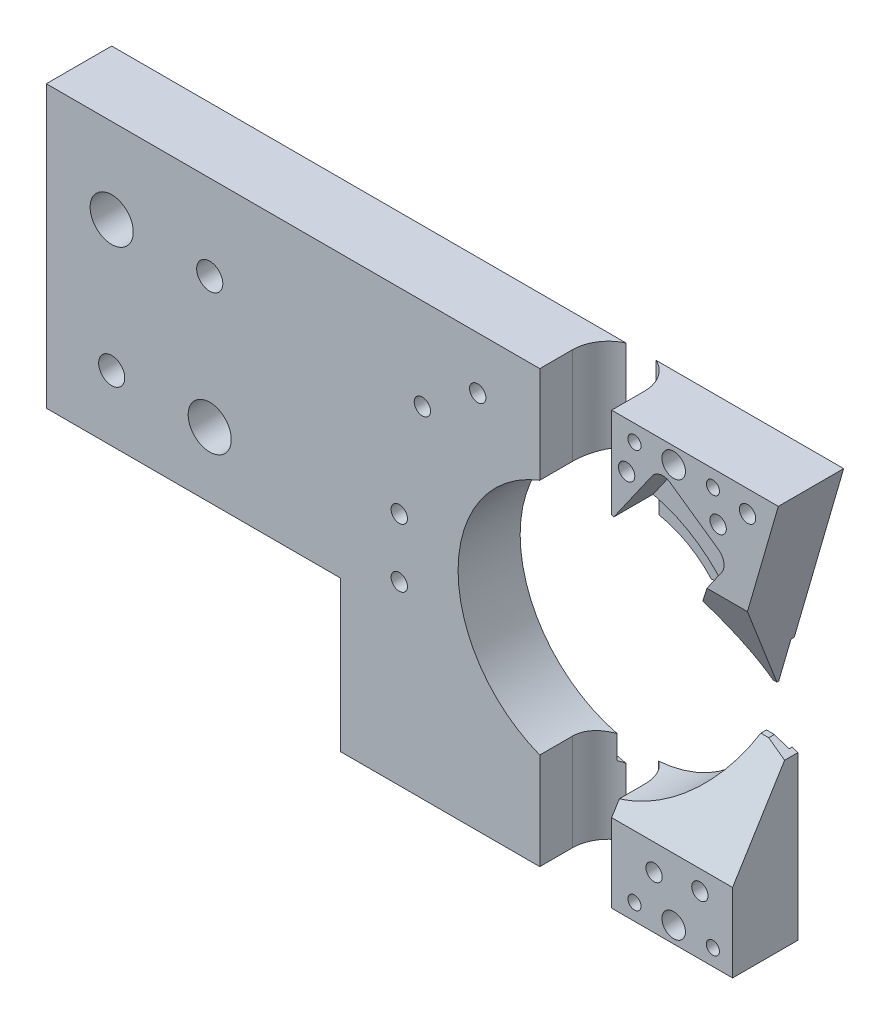
SolidWorks part; units mm, degrees
ref_plane "前视基准面" through (0, 0, 0) normal (0, 0, 1) x (1, 0, 0)
ref_plane "上视基准面" through (0, 0, 0) normal (0, 1, 0) x (1, 0, 0)
ref_plane "右视基准面" through (0, 0, 0) normal (1, 0, 0) x (0, 0, -1)
sketch "草图1" plane through (0, 0, 0) normal (0, 0, 1) x (1, 0, 0)
  line L0 (-53.8847, 0) -> (-8.8847, 0)
  line L1 (-53.8847, 43) -> (58.1153, 43)
  line L2 (-53.8847, 43) -> (-53.8847, 0)
  line L3 (-8.8847, -23) -> (58.1153, -23)
  line L4 (58.1153, 43) -> (58.1153, -23)
  line L5 (-8.8847, 0) -> (-8.8847, -23)
  dimension "D1" = 66
  dimension "D5" = 45
  dimension "D6" = 23
extrude "凸台-拉伸1" add sketch "草图1" along normal blind 10
sketch "草图3" plane through (0, -23, 0) normal (0, -1, 0) x (1, 0, 0)
  line L0 (32.6153, 5) -> (32.6153, 10)
  line L1 (-8.8847, 10) -> (58.1153, 10) construction
  line L3 (21.6153, 10) -> (21.6153, 5)
  line L4 (32.6153, 10) -> (21.6153, 10)
  line L5 (58.1153, 10) -> (58.1153, 0) construction
  arc A0 (21.6153, 5) -> (32.6153, 5) centre (27.1153, 5) ccw
  dimension "D1" = 5.5
  dimension "D2" = 5
  dimension "D3" = 25.5
extrude "切除-拉伸2" cut sketch "草图3" against normal through all
sketch "草图4" plane through (0, 0, 0) normal (0, 0, -1) x (-1, 0, 0)
  line L0 (-58.1153, -23) -> (-58.1153, 43)
  line L1 (-58.1153, -23) -> (-51.1153, -23)
  line L2 (-29.4066, -23) -> (-58.1153, -23) construction
  line L3 (-51.1153, -23) -> (-51.1153, 1.87)
  line L4 (-51.1153, 1.87) -> (-44.4875, 4.2199)
  line L5 (-44.4875, 4.2199) -> (-45.4997, 10)
  line L6 (-45.4997, 10) -> (-48.4191, 9.4887)
  line L7 (-48.4191, 9.4887) -> (-58.1153, 43)
  dimension "D1" = 7
  dimension "D2" = 24.87
extrude "切除-拉伸3" cut sketch "草图4" against normal through all
ref_plane "基准面4" through (80, 0, 0) normal (1, 0, 0) x (0, 0, -1)
sketch "草图6" plane through (80, 0, 0) normal (1, 0, 0) x (0, 0, -1)
  line L0 (-10, 26.69) -> (-0.78, 10.37)
  line L1 (-0.78, 10.37) -> (0, 10.37)
  line L2 (0, 10.37) -> (0, 2.97)
  line L3 (0, 2.97) -> (-1.36, 2.97)
  line L4 (-1.36, 2.97) -> (-10, -11)
  line L5 (-10, -11) -> (-10, 26.69)
extrude "切除-拉伸4" cut sketch "草图6" against normal blind 56
sketch "草图7" plane through (0, 0, 0) normal (0, 0, -1) x (-1, 0, 0)
  line L0 (53.8847, 43) -> (53.8847, 0) construction
  line L1 (-29.4066, -23) -> (-51.1153, -23) construction
  circle A0 centre (-28.6153, 10) radius 23
  dimension "D1" = 46
  dimension "D2" = 82.5
  dimension "D3" = 33
extrude "切除-拉伸5" cut sketch "草图7" against normal blind 0.5
sketch "草图8" plane through (0, 0, 10) normal (0, 0, 1) x (1, 0, 0)
  line L0 (-8.8847, -23) -> (21.6153, -23) construction
  line L1 (-53.8847, 43) -> (-53.8847, 0) construction
  circle A0 centre (28.6153, 10) radius 19.5
  point P6 (-53.8847, 21.5)
  dimension "D1" = 39
  dimension "D2" = 33
  dimension "D3" = 82.5
extrude "切除-拉伸6" cut sketch "草图8" against normal blind 8.5
sketch "草图9" plane through (0, 0, 0) normal (0, 0, -1) x (-1, 0, 0)
  line L1 (-39.3596, 19.737) -> (-45.0697, 20.4642)
  line L4 (-30.6379, 29.3948) -> (-30.6379, 24.3582)
  arc A0 (-45.0697, 20.4642) -> (-30.6379, 29.3948) centre (-28.6153, 10) ccw
  arc A3 (-30.6379, 24.3582) -> (-39.3596, 19.737) centre (-28.6153, 10) ccw
  dimension "D1" = 39
extrude "切除-拉伸7" cut sketch "草图9" against normal blind 8
sketch "草图10" plane through (0, 0, 0) normal (0, 0, -1) x (-1, 0, 0)
  line L0 (53.8847, 43) -> (53.8847, 0) construction
  line L1 (53.8847, 0) -> (8.8847, 0) construction
  line L2 (8.8847, 0) -> (8.8847, -23) construction
  line L3 (-24.824, 43) -> (53.8847, 43) construction
  line L4 (-23.953, 32.5225) -> (-23.953, 28.9344) construction
  line L5 (-24.824, 43) -> (-24.824, 32.6854) construction
  line L6 (-29.4066, -23) -> (-29.4066, -12.9864) construction
  line L7 (-29.4066, -23) -> (-51.1153, -23) construction
  line L8 (-51.1153, -23) -> (-51.1153, 1.87) construction
  line L9 (-29.4066, 32.9864) -> (-29.4066, 43) construction
  line L10 (-58.1153, 43) -> (-29.4066, 43) construction
  line L11 (-30.2775, 29.429) -> (-30.2775, 32.9399) construction
  circle A0 centre (43.8847, 10) radius 2
  circle A1 centre (28.8847, 10) radius 3.3
  circle A2 centre (28.8847, 30) radius 2
  circle A3 centre (43.8847, 30) radius 3.3
  circle A4 centre (-0.1153, 4) radius 1.25
  circle A5 centre (-0.1153, 13) radius 1.25
  circle A6 centre (-3.653, 29) radius 1.25
  circle A7 centre (-12.124, 35) radius 1.25
  circle A8 centre (-48.1066, -20.5) radius 1
  circle A9 centre (-42.1066, -20.5) radius 1.8
  circle A10 centre (-36.1066, -20.5) radius 1
  circle A11 centre (-46.1153, -14) radius 1.25
  circle A12 centre (-39.1066, -14.9964) radius 1.25
  circle A13 centre (-34.9066, 36) radius 1.25
  circle A14 centre (-36.1066, 40.5) radius 1
  circle A15 centre (-41.4066, 34.9911) radius 0.8
  circle A16 centre (-42.1066, 40.5) radius 1.8
  circle A17 centre (-48.9066, 36) radius 1.25
  circle A18 centre (-46.4775, 31.5) radius 0.8
  circle A19 centre (-48.1066, 40.5) radius 1
  circle A21 centre (-53.4066, 39.65) radius 1.25
  point P66 (-29.4066, 32.9911)
  dimension "D12" = 2.5
  dimension "D13" = 2.5
  dimension "D14" = 2.5
  dimension "D15" = 2.5
  dimension "D29" = 6.6
  dimension "D30" = 4
  dimension "D31" = 6.6
  dimension "D32" = 4
  dimension "D33" = 2
  dimension "D34" = 3.6
  dimension "D35" = 2
  dimension "D36" = 2.5
  dimension "D37" = 2.5
  dimension "D38" = 2.5
  dimension "D39" = 2
  dimension "D48" = 1.6
  dimension "D49" = 3.6
  dimension "D54" = 2
  dimension "D55" = 2.5
  dimension "D58" = 1.6
  dimension "D63" = 2.5
  dimension "D1" = 10
  dimension "D2" = 15
  dimension "D4" = 10
  dimension "D6" = 15
  dimension "D7" = 10
  dimension "D8" = 9
  dimension "D9" = 4
  dimension "D10" = 9
  dimension "D11" = 0
  dimension "D16" = 14
  dimension "D17" = 20.3
  dimension "D18" = 8
  dimension "D19" = 12.7
  dimension "D20" = 6.7
  dimension "D21" = 2.5
  dimension "D22" = 0
  dimension "D23" = 6
  dimension "D24" = 0
  dimension "D25" = 6
  dimension "D26" = 9.7
  dimension "D27" = 5
  dimension "D28" = 9
  dimension "D40" = 5.5
  dimension "D41" = 7
  dimension "D42" = 6.7
  dimension "D43" = 2.5
  dimension "D44" = 0
  dimension "D45" = 6
  dimension "D46" = 2
  dimension "D47" = 12
  dimension "D50" = 2.5
  dimension "D51" = 18.7
  dimension "D52" = 7
  dimension "D53" = 19.5
  dimension "D56" = 11.5
  dimension "D57" = 16.2
  dimension "D59" = 3.35
  dimension "D60" = 24
  dimension "D65" = 10
  dimension "D66" = 13
  dimension "D67" = 13
extrude "切除-拉伸8" cut sketch "草图10" against normal through all
sketch "草图11" plane through (0, 0, 10) normal (0, 0, 1) x (1, 0, 0)
  line L0 (28.6153, 10) -> (28.6153, 48.882)
  line L2 (32.9487, 29.0124) -> (38.7992, 37.3677)
  line L5 (41.5847, 37.8589) -> (48.957, 32.6967)
  line L7 (49.4482, 29.9112) -> (43.945, 22.0519)
  arc A0 (43.945, 22.0519) -> (32.9487, 29.0124) centre (28.6153, 10) ccw
  arc A1 (41.5847, 37.8589) -> (38.7992, 37.3677) centre (40.4375, 36.2206) ccw
  arc A2 (49.4482, 29.9112) -> (48.957, 32.6967) centre (47.8099, 31.0584) ccw
  dimension "D2" = 10.2
  dimension "D5" = 2
extrude "切除-拉伸9" cut sketch "草图11" against normal blind 6
